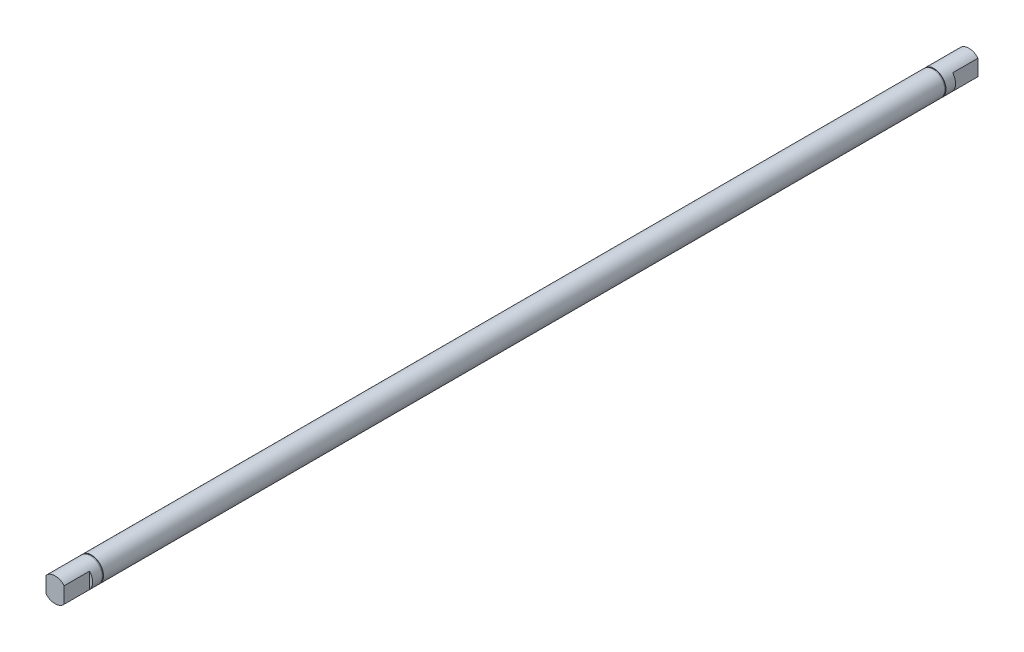
SolidWorks part; units mm, degrees
material "普通碳钢"
ref_plane "前视基准面" through (0, 0, 0) normal (0, 0, 1) x (1, 0, 0)
ref_plane "上视基准面" through (0, 0, 0) normal (0, 1, 0) x (1, 0, 0)
ref_plane "右视基准面" through (0, 0, 0) normal (1, 0, 0) x (0, 0, -1)
sketch "草图1" plane through (0, 0, 0) normal (0, 0, 1) x (1, 0, 0)
  circle A0 centre (0, 0) radius 10
  dimension "D1" = 20
extrude "凸台-拉伸1" add sketch "草图1" along normal mid plane 755
sketch "草图2" plane through (0, 0, 0) normal (0, 1, 0) x (1, 0, 0)
  line L0 (0, 0) -> (0, 99.7589) construction
  line L1 (-28.4039, 377.5) -> (-7.5, 377.5)
  line L2 (-28.4039, 377.5) -> (-28.4039, 356.5)
  line L3 (-28.4039, 356.5) -> (-7.5, 356.5)
  line L4 (-7.5, 377.5) -> (-7.5, 356.5)
  line L5 (0, 0) -> (39.8976, 0) construction
  line L6 (7.5, 377.5) -> (7.5, 356.5)
  line L7 (28.4039, 356.5) -> (7.5, 356.5)
  line L8 (28.4039, 377.5) -> (28.4039, 356.5)
  line L9 (28.4039, 377.5) -> (7.5, 377.5)
  line L10 (28.4039, -377.5) -> (7.5, -377.5)
  line L11 (28.4039, -377.5) -> (28.4039, -356.5)
  line L12 (28.4039, -356.5) -> (7.5, -356.5)
  line L13 (7.5, -377.5) -> (7.5, -356.5)
  line L14 (-7.5, -377.5) -> (-7.5, -356.5)
  line L15 (-28.4039, -356.5) -> (-7.5, -356.5)
  line L16 (-28.4039, -377.5) -> (-28.4039, -356.5)
  line L17 (-28.4039, -377.5) -> (-7.5, -377.5)
  line L18 (10, 377.5) -> (-10, 377.5) construction
  dimension "D1" = 15
  dimension "D2" = 21
extrude "切除-拉伸1" cut sketch "草图2" against normal mid plane 50
ref_plane "基准面1" through (0, 20, 0) normal (0, 1, 0) x (1, 0, 0)
sketch "草图5" plane through (0, 0, -377.5) normal (0, 0, -1) x (-1, 0, 0)
  circle A0 centre (0, 0) radius 9.5
  circle A2 centre (0, 0) radius 10
  circle A3 centre (0, 0) radius 10
  dimension "D2" = 19
  dimension "D1" = 0
extrude "切除-拉伸2" cut sketch "草图5" along normal blind 1.1 from offset 30 offset against normal yes
mirror "镜向1" about plane through (0, 0, 0) normal (0, 0, 1) of "切除-拉伸2"
